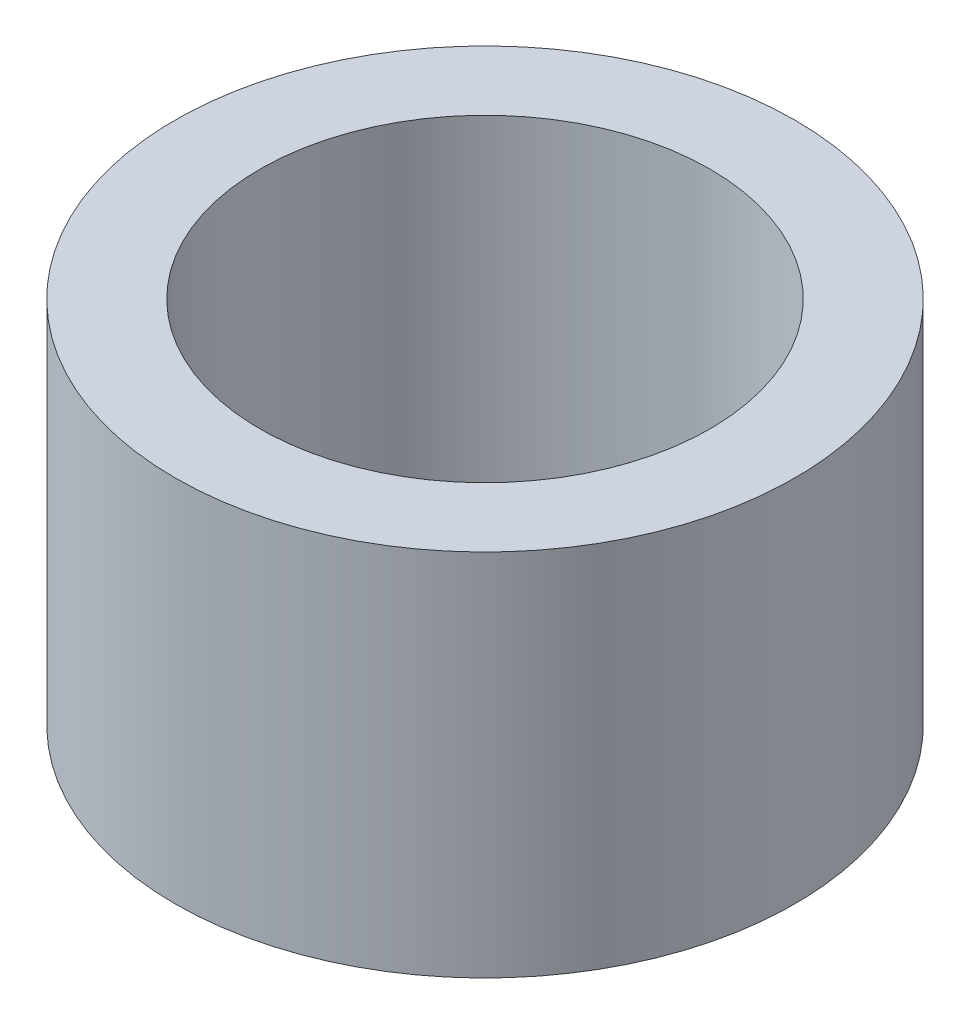
SolidWorks part; units mm, degrees
material "S45C"
ref_plane "Front Plane" through (0, 0, 0) normal (0, 0, 1) x (1, 0, 0)
ref_plane "Top Plane" through (0, 0, 0) normal (0, 1, 0) x (1, 0, 0)
ref_plane "Right Plane" through (0, 0, 0) normal (1, 0, 0) x (0, 0, -1)
sketch "Sketch1" plane through (0, 0, 0) normal (0, 0, 1) x (1, 0, 0)
  line L0 (0, 0) -> (0, 23.4621) construction
  line L1 (3.05, 2.5) -> (4.2, 2.5)
  line L2 (3.05, 2.5) -> (3.05, -2.5)
  line L3 (3.05, -2.5) -> (4.2, -2.5)
  line L4 (4.2, 2.5) -> (4.2, -2.5)
  line L5 (3.05, 2.5) -> (4.2, -2.5) construction
  line L6 (3.05, -2.5) -> (4.2, 2.5) construction
  point P0 (3.625, 0)
  dimension "D1" = 3.05
  dimension "D2" = 5
  dimension "D3" = 4.2
revolve "Revolve1" add sketch "Sketch1" angle 360 about L0
